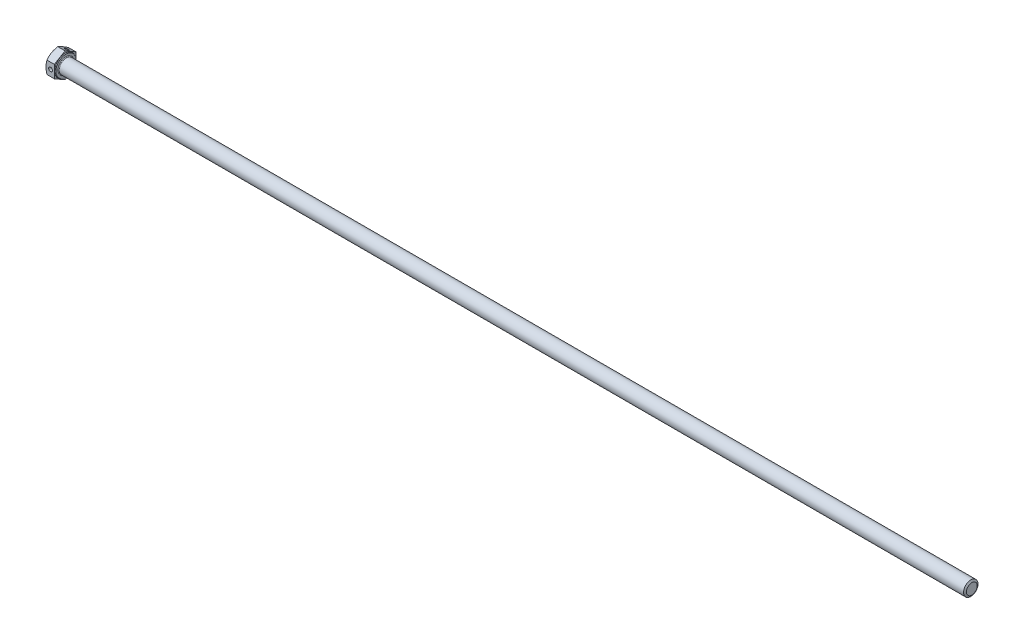
from build123d import *

# Parameters (mm, degrees)
EXTRUDE_405_DEPTH        = 7.5
FILLET_1252_R            = 0.6
SKETCH_7_R               = 1.6
CUT_EXTRUDE_1_DEPTH      = 761.624250205
PATTERN_CIRCULAR_1_COUNT = 2
PATTERN_CIRCULAR_1_ANGLE = 60


with BuildPart() as part:
    # 草图1 → Extrude 405 (new body)
    with BuildSketch(Plane(origin=(0, 0, 0), x_dir=(0, 0, -1), z_dir=(1, 0, 0))):
        Polygon((9, 5.196152423), (9, -5.196152423), (0, -10.392304845), (-9, -5.196152423), (-9, 5.196152423), (0, 10.392304845), align=None)
    extrude(amount=EXTRUDE_405_DEPTH)

    # 草图2 → 凸台-旋转1 (revolve)
    with BuildSketch(Plane.XY, mode=Mode.PRIVATE) as revolve_1_sk:
        Polygon((0, 0), (760.5, 0), (760.5, 4.4845), (760.5, 6), (730.5, 6), (0, 6), align=None)
    revolve(revolve_1_sk.sketch.rotate(Axis((0, 0, 0), (1, 0, 0)), 90), axis=Axis((0, 0, 0), (1, 0, 0)))

    # 草图3 → 切除-旋转1 (revolve, cut)
    with BuildSketch(Plane.XY):
        Polygon((0, 9), (3.690598923, 15.392304845), (3.690598923, 20.392304845), (-10, 20.392304845), (-10, 9), align=None)
    revolve(axis=Axis((0, 0, 0), (1, 0, 0)), mode=Mode.SUBTRACT)

    # 草图5 → 切除-旋转5 (revolve, cut)
    with BuildSketch(Plane.XY, mode=Mode.PRIVATE) as cut_revolve_5_sk:
        Polygon((7.5, 8.315), (6.9, 8.661410162), (6.9, 10.392304845), (7.5, 10.392304845), align=None)
    revolve(cut_revolve_5_sk.sketch.rotate(Axis((0, 0, 0), (1, 0, 0)), 180), axis=Axis((0, 0, 0), (1, 0, 0)), mode=Mode.SUBTRACT)

    # Fillet 1252
    fillet_1252_edges = [part.edges().sort_by_distance(p)[0] for p in [
        (7.5, 0, -6),
    ]]
    fillet(fillet_1252_edges, radius=FILLET_1252_R)

    # 草图6 → 切除-旋转4 (revolve, cut)
    with BuildSketch(Plane.XY, mode=Mode.PRIVATE) as cut_revolve_4_sk:
        Polygon((759.625, 6), (761.375, 6), (760.5, 4.484455543), align=None)
    revolve(cut_revolve_4_sk.sketch.rotate(Axis((0, 0, 0), (1, 0, 0)), 90), axis=Axis((0, 0, 0), (1, 0, 0)), mode=Mode.SUBTRACT)

    # 草图7 → 切除-拉伸1 (cut, symmetric)
    with BuildSketch(Plane.XY):
        with Locations((3.8, 0)):
            Circle(SKETCH_7_R)
    cut_extrude_1 = extrude(amount=CUT_EXTRUDE_1_DEPTH, both=True, mode=Mode.SUBTRACT)

    # 阵列(圆周)1: 切除-拉伸1 ×2 about axis
    pattern_circular_1_axis = Axis((0, 0, 0), (1, 0, 0))
    for i in range(1, PATTERN_CIRCULAR_1_COUNT):
        add(cut_extrude_1.rotate(pattern_circular_1_axis, i * PATTERN_CIRCULAR_1_ANGLE / (PATTERN_CIRCULAR_1_COUNT - 1)), mode=Mode.SUBTRACT)


solid = part.part
